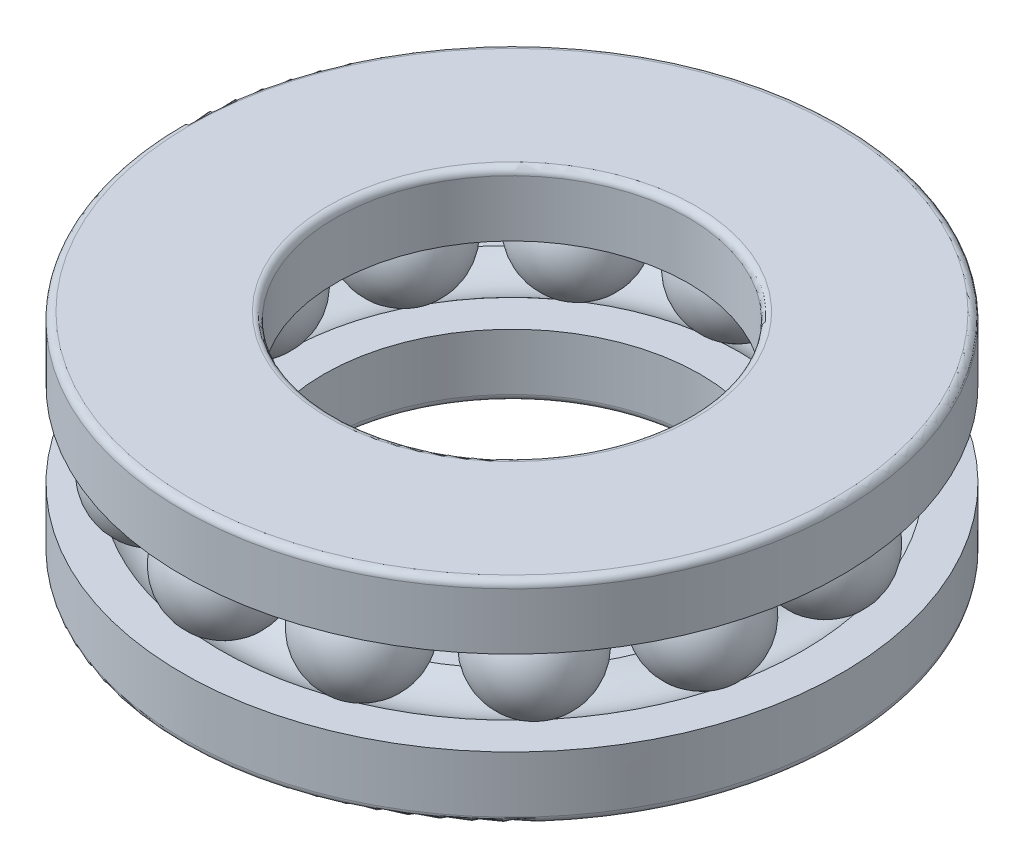
from build123d import *

# Parameters (mm, degrees)
CIRPATTERN1_COUNT = 13
FILLET1_R         = 0.3


with BuildPart() as part:
    # Sketch2 → Base-Revolve (revolve)
    with BuildSketch(Plane.XY, mode=Mode.PRIVATE) as base_revolve_sk:
        with BuildLine():
            Line((0, 2.7), (1.65, 2.7))
            ThreePointArc((1.65, 2.7), (3, 2.25), (4.35, 2.7))
            Line((4.35, 2.7), (6, 2.7))
            Line((6, 2.7), (6, 0))
            Line((6, 0), (0, 0))
            Line((0, 0), (0, 2.7))
        make_face()
    revolve(base_revolve_sk.sketch.rotate(Axis((14, 0, 0), (0, 1, 0)), 270), axis=Axis((14, 0, 0), (0, 1, 0)))

    # Sketch3 → Boss-Revolve2 (revolve)
    with BuildSketch(Plane.XY):
        with BuildLine():
            Line((3, 2.2), (3, 6.8))
            ThreePointArc((3, 6.8), (0.7, 4.5), (3, 2.2))
        make_face()
    boss_revolve2 = revolve(axis=Axis((3, 0, 0), (0, 1, 0)))

    # Sketch4 → Boss-Revolve3 (revolve)
    with BuildSketch(Plane.XY, mode=Mode.PRIVATE) as boss_revolve3_sk:
        with BuildLine():
            Line((0, 6.3), (1.65, 6.3))
            ThreePointArc((1.65, 6.3), (3, 6.75), (4.35, 6.3))
            Line((4.35, 6.3), (6.5, 6.3))
            Line((6.5, 6.3), (6.5, 9))
            Line((6.5, 9), (0, 9))
            Line((0, 9), (0, 6.3))
        make_face()
    revolve(boss_revolve3_sk.sketch.rotate(Axis((14, 0, 0), (0, 1, 0)), 270), axis=Axis((14, 0, 0), (0, 1, 0)))

    # CirPattern1: Boss-Revolve2 ×13 about axis
    cirpattern1_axis = Axis((14, 0, 0), (0, 1, 0))
    for i in range(1, CIRPATTERN1_COUNT):
        add(boss_revolve2.rotate(cirpattern1_axis, i * 360 / CIRPATTERN1_COUNT))

    # Fillet1
    fillet1_edges = [part.edges().sort_by_distance(p)[0] for p in [
        (14, 9, 7.5),
        (14, 9, 14),
        (14, 0, 8),
        (14, 0, 14),
    ]]
    fillet(fillet1_edges, radius=FILLET1_R)


solid = part.part
